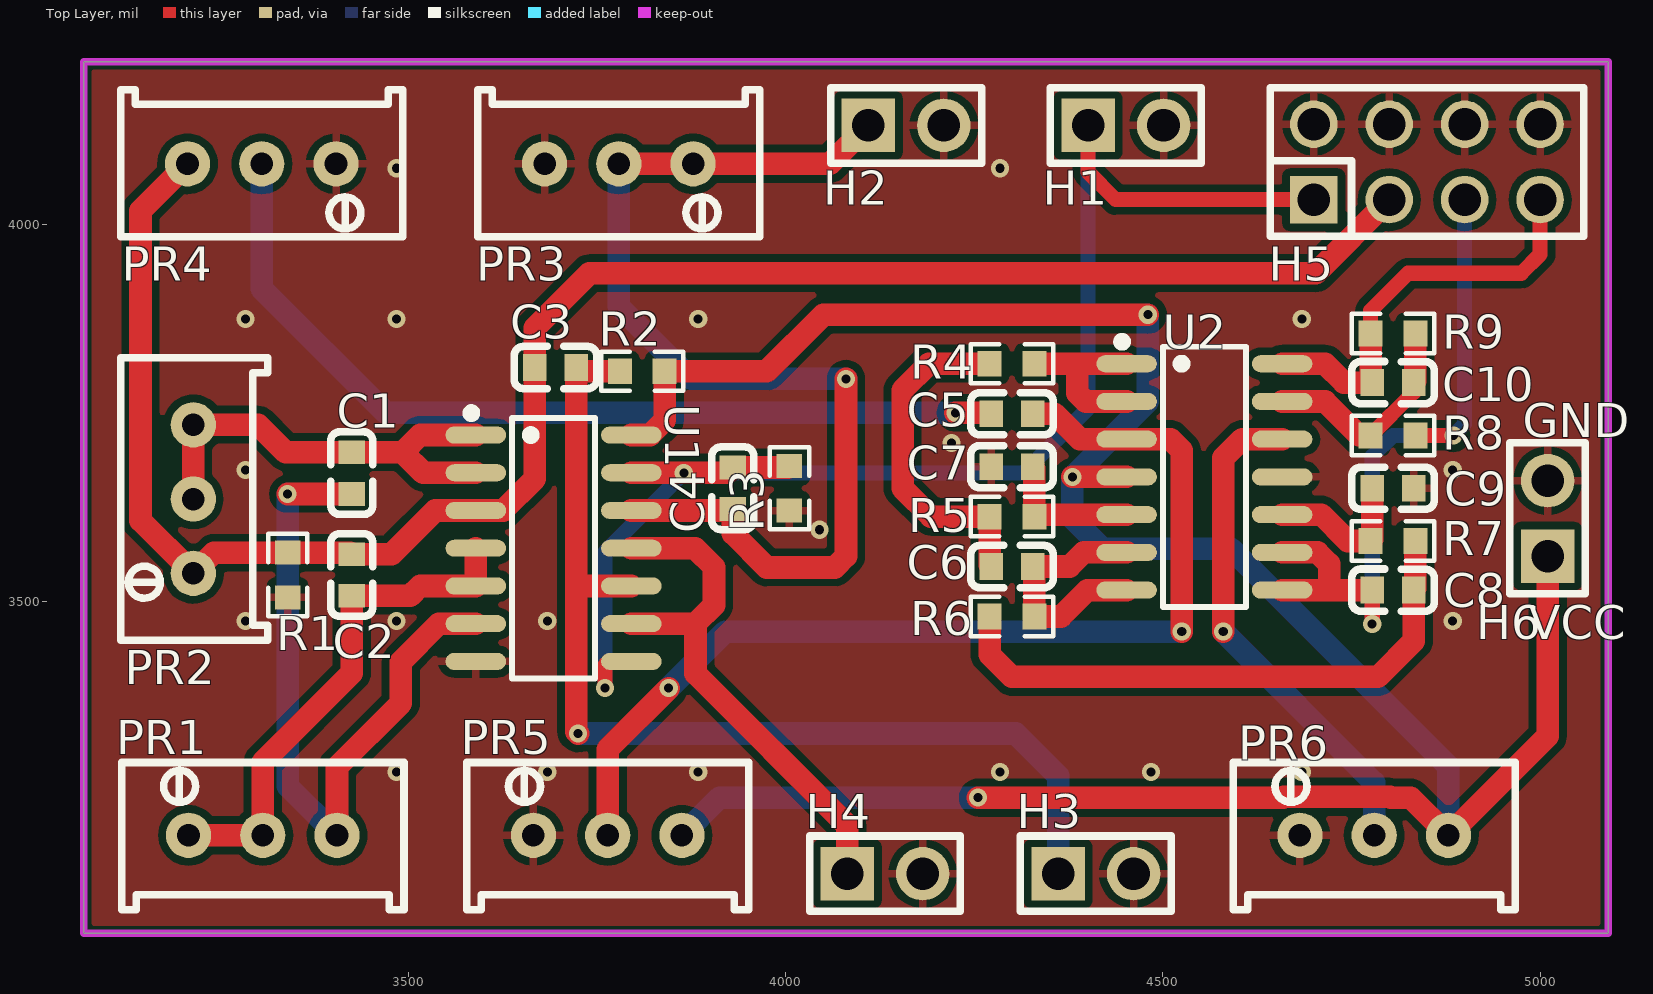
[diagram p0: Top Layer view]
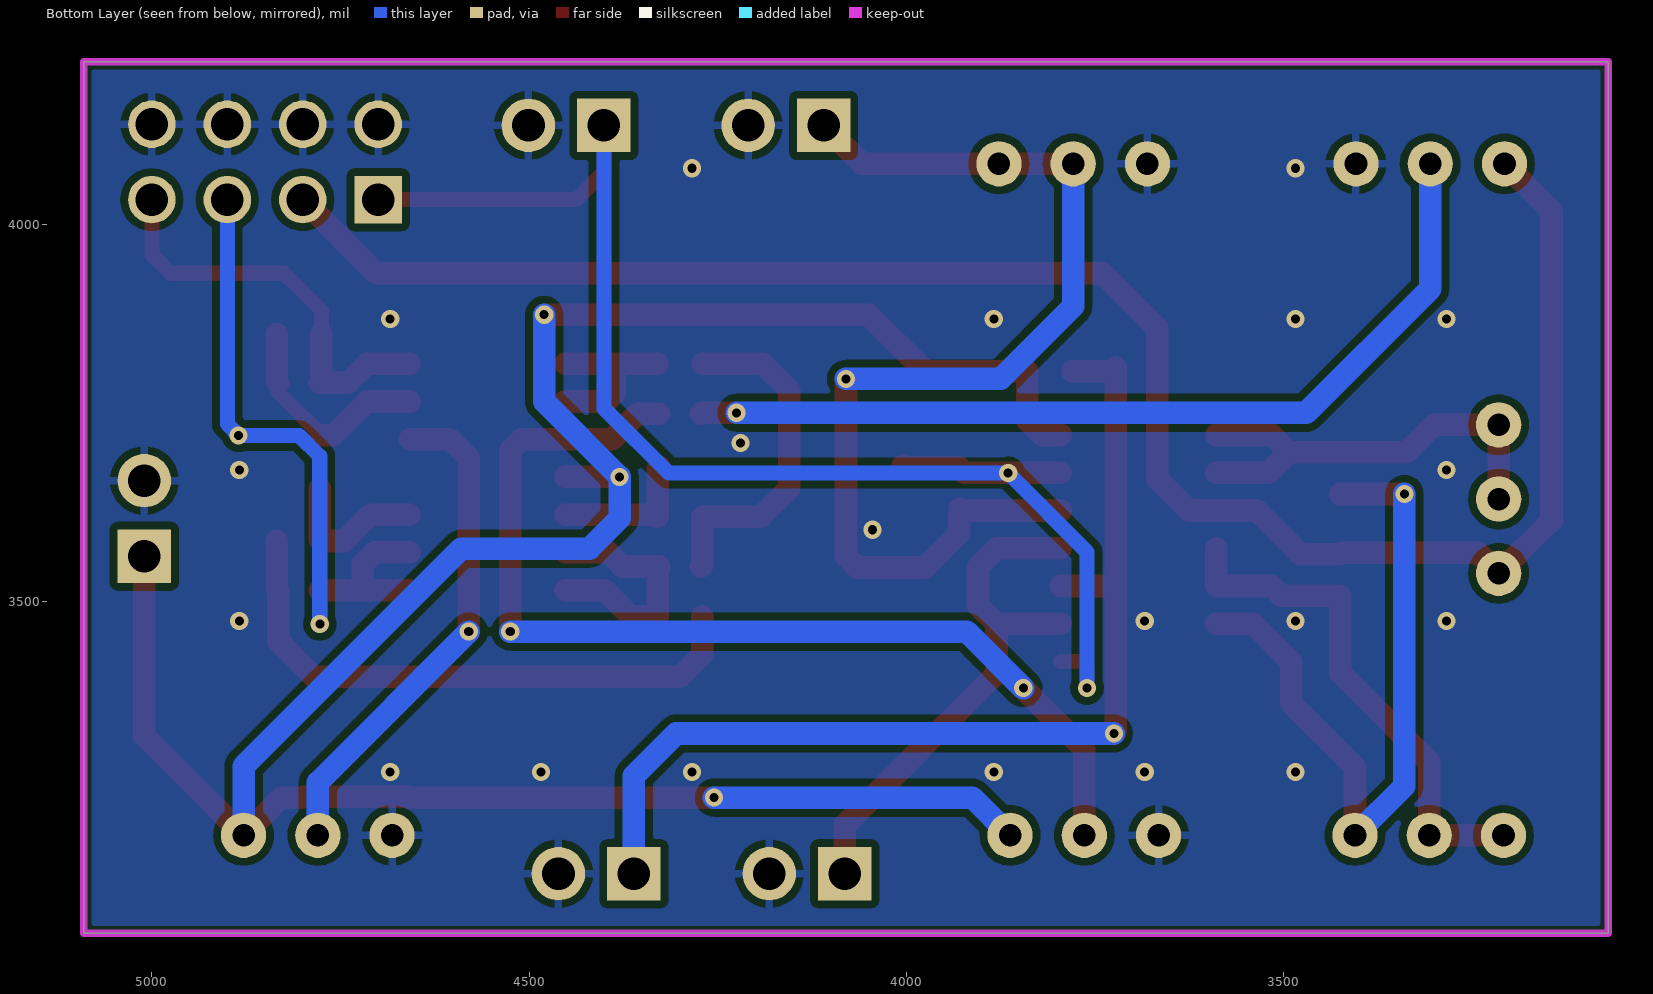
[diagram p1: Bottom Layer view, seen from below]
# Altium PCB MISC89095.pcbdoc
Units mil, origin at the board's own origin, x right, y up, seen from the top; angles counter-clockwise.
Board outline 2020 x 1155 mil, 2 copper layers (Top Layer, Bottom Layer), stack 62.206 mil thick; 33 components, 22 nets, 102 pads, 34 vias.

## Layer stack, top to bottom
Top Solder Mask Layer: solder mask 0.394, Dk 3.3
Top Layer: signal copper 1.379
Dielectric1: surface 59.449, FR4, Dk 4.5
Bottom Layer: signal copper 1.378
Bottom Solder Mask Layer: solder mask 0.394, Dk 3.3

## Board outline
3070,4215 3070,3060 5090,3060 5090,4215

## Design rules (kind name [scope] priority, off if disabled: settings)
BoardOutlineClearance copperThickness2oz_1 [All] p2 off: genericclearance=7.99 ignorepadtopadclearanceinfootprint=FALSE except(0: Arc-SplitContinuation Track-SplitContinuation SMDPad-SplitContinuation THPad-SplitContinuation Via-SplitContinuation Fill-SplitContinuation Region-SplitContinuation Poly-SplitContinuation Text-SplitContinuation Hole-SplitContinuation; 5.98: Arc-CutoutEdge SMDPad-CutoutEdge THPad-CutoutEdge Via-CutoutEdge Fill-CutoutEdge Region-CutoutEdge Text-CutoutEdge; 6.93: Hole-OutlineEdge Hole-CutoutEdge; 10: Poly-OutlineEdge Poly-CutoutEdge; 11.81: Arc-OutlineEdge Track-OutlineEdge SMDPad-OutlineEdge THPad-OutlineEdge Via-OutlineEdge Fill-OutlineEdge Region-OutlineEdge Text-OutlineEdge Track-CutoutEdge)
BoardOutlineClearance copperThickness1oz_1 [All] p4: genericclearance=4.02 ignorepadtopadclearanceinfootprint=FALSE except(0: Arc-SplitContinuation Track-SplitContinuation SMDPad-SplitContinuation THPad-SplitContinuation Via-SplitContinuation Fill-SplitContinuation Region-SplitContinuation Poly-SplitContinuation Text-SplitContinuation Hole-SplitContinuation; 6: SMDPad-CutoutEdge THPad-CutoutEdge Via-CutoutEdge Fill-CutoutEdge Region-CutoutEdge Text-CutoutEdge; 6.93: Hole-OutlineEdge Hole-CutoutEdge; 10: Poly-OutlineEdge Poly-CutoutEdge; 11.8: Arc-OutlineEdge Track-OutlineEdge SMDPad-OutlineEdge THPad-OutlineEdge Via-OutlineEdge Fill-OutlineEdge Region-OutlineEdge Text-OutlineEdge; 11.81: Arc-CutoutEdge Track-CutoutEdge)
Clearance copperThickness2oz [All] p1 off: gap=7.99 ignorepadtopadclearanceinfootprint=FALSE except(5.98: SMDPad-Track SMDPad-SMDPad THPad-Track SMDPad-THPad THPad-THPad Track-Via SMDPad-Via THPad-Via Via-Via Fill-Track Region-Track Fill-SMDPad Region-SMDPad Fill-THPad Region-THPad Fill-Via Region-Via Fill-Fill Fill-Region Region-Region Arc-Track Arc-SMDPad Arc-THPad Arc-Via Fill-Arc Region-Arc Arc-Arc Text-Track SMDPad-Text Text-THPad Text-Via Fill-Text Region-Text Arc-Text Text-Text; 6.93: Hole-Track Hole-SMDPad Hole-THPad Hole-Via Fill-Hole Region-Hole Hole-Arc Hole-Text; 10: Poly-Track Poly-SMDPad Poly-THPad Poly-Via Poly-Fill Poly-Region Poly-Poly Poly-Arc Poly-Text Poly-Hole)
Clearance copperThickness1oz [All] p3: gap=4.02 ignorepadtopadclearanceinfootprint=FALSE except(5.98: SMDPad-Track SMDPad-SMDPad THPad-Track SMDPad-THPad THPad-THPad Track-Via SMDPad-Via THPad-Via Via-Via Fill-Track Region-Track Fill-SMDPad Region-SMDPad Fill-THPad Region-THPad Fill-Via Region-Via Fill-Fill Fill-Region Region-Region; 6: Arc-Track Arc-SMDPad Arc-THPad Arc-Via Fill-Arc Region-Arc Arc-Arc Text-Track SMDPad-Text Text-THPad Text-Via Fill-Text Region-Text Arc-Text Text-Text; 6.93: Hole-Track Hole-SMDPad Hole-THPad Hole-Via Fill-Hole Region-Hole Hole-Arc Hole-Text; 10: Poly-Track Poly-SMDPad Poly-THPad Poly-Via Poly-Fill Poly-Region Poly-Poly Poly-Arc Poly-Text Poly-Hole)
Creepage creepage [All] p1: checkdistance=0 ignoreinternallayers=TRUE applytopolygonpour=TRUE
DiffPairsRouting differentialPair [All] p1: maxlimit=6 minlimit=6 mostfreqgap=6 toplayer_minwidth=5 toplayer_prefwidth=10 toplayer_maxwidth=100 toplayer_mingap=6 toplayer_prefgap=6 toplayer_maxgap=6 bottomlayer_minwidth=5 bottomlayer_prefwidth=10 bottomlayer_maxwidth=100 bottomlayer_mingap=6 bottomlayer_prefgap=6 bottomlayer_maxgap=6 maxuncoupledlength=10
HoleToHoleClearance otherClearance [All] p1: gap=11.81 allowstackedmicrovias=TRUE
Length netLength [All] p1: minlimit=0 maxlimit=0
MatchedLengths netLengthTolerance [All] p1: tolerance=1000
PasteMaskExpansion pasteMaskExpansion [All] p1: expansion=0
PlaneConnect innerPlane [All] p1: planeconnectstyle=Relief reliefexpansion=20 reliefentries=4 reliefconductorwidth=10 reliefairgap=10
PolygonConnect copperRegion [(InNet('GND'))] p1: connectstyle=Relief reliefconductorwidth=10 reliefentries=4 polygonreliefangle="90 Angle" airgapwidth=10 via.connectstyle=Relief via.reliefconductorwidth=10 via.reliefentries=4 via.polygonreliefangle="90 Angle" via.airgapwidth=10
RoutingVias viaSize [All] p1: holewidth=12.01 width=24.02 viastyle="Through Hole" minholewidth=11.81 minwidth=19.68 maxholewidth=248.03 maxwidth=393.7
SolderMaskExpansion solderMaskExpansion [IsVia] p1: expansion=-1000 istentingtop=TRUE
SolderMaskExpansion solderMaskExpansion [All] p2: expansion=2 istentingtop=FALSE
Width copperThickness2oz_2 [All] p1 off: maxlimit=100 minlimit=8 preferedwidth=10
Width copperThickness1oz_2 [All] p2: maxlimit=100 minlimit=5 preferedwidth=10

## Components (designator, comment, footprint, x,y, rotation, side; value= is the part's Value field where it differs from the comment)
C1 "22nF" C0603 3425,3670 r270 top
C2 "22nF" C0603 3425,3535 r270 top
C3 "100PF" C0603 3695,3810 r0 top
C4 "1nF" C0603 3930,3650 r90 top
C5 "100nF" C0603 4300,3748.79 r0 top
C6 "100pF" C0603 4300,3546.21 r0 top
C7 "100pF" C0603 4300,3678.63 r0 top
C8 "100pF" C0603 4805,3515 r180 top
C9 "80pF" C0603 4805,3650 r180 top
C10 "500pF" C0603 4805,3790 r0 top
H1 "" HDR-TH_2P-P2.54-V-M-1 4450.89,4130.9 r0 top
H2 "" HDR-TH_2P-P2.54-V-M-1 4159.66,4130.9 r0 top
H3 "" HDR-TH_2P-P2.54-V-M-1 4411.1,3139.1 r0 top
H4 "" HDR-TH_2P-P2.54-V-M-1 4131.7,3139.1 r0 top
H5 "" HDR-TH_8P-P2.54-V-F-R2-C4-S2.54-1 4850,4082.47 r0 top
H6 "" HDR-TH_2P-P2.54-V-M-1 5010,3610 r90 top
PR1 "10kΩ" R_3296 3307,3195 r0 top
PR2 "10kΩ" R_3296 3210,3635.65 r90 top
PR3 "20kΩ" R_3296 3778.93,4075 r180 top
PR4 "10kΩ" R_3296 3305.7,4075 r180 top
PR5 "10kΩ" R_3296 3764.1,3195 r0 top
PR6 "100kΩ" R_3296 4780,3195 r0 top
R1 "1K" R0603 3340,3535 r90 top
R2 "10K" R0603 3810,3805 r0 top
R3 "1K" R0603 4005,3650 r90 top
R4 "100K" R0603 4300,3815 r180 top
R5 "100K" R0603 4300,3612.42 r0 top
R6 "200K" R0603 4300,3480 r180 top
R7 "100K" R0603 4805,3580 r180 top
R8 "40K" R0603 4805,3720 r180 top
R9 "100K" R0603 4805,3855 r180 top
U1 "SN74LS00DG4" SOIC-14_L8.7-W3.9-P1.27-LS6.0-BL 3692.45,3570.51 r270 top
U2 "LM324DT" SOIC-14_L8.7-W3.9-P1.27-LS6.0-BL 4555,3665 r270 top

## Footprints (in the part's own frame and the unit in brackets; to place one, negate y for a bottom-side part, rotate by r counter-clockwise, add the part's x,y. Pads: shape width x height; smd on the part's side, far side on the other; paste and mask are expansions set on the pad)
C0603 [mm]
  rect 0.8x0.9 smd: 1(-0.7,0) 2(0.7,0)
  silkscreen extent -1.39,-0.71 1.39,0.71
HDR-TH_2P-P2.54-V-M-1 [mm]
  rect 1.8x1.8 hole 1.1: 1(-1.27,0)
  round 1.8 hole 1.1: 2(1.27,0)
  silkscreen extent -2.54,-1.27 2.54,1.27
HDR-TH_8P-P2.54-V-F-R2-C4-S2.54-1 [mm]
  rect 1.6x1.6 hole 1.1: 1(-3.81,-1.27)
  round 1.6 hole 1.1: 2(-3.81,1.27) 3(-1.27,-1.27) 4(-1.27,1.27) 5(1.27,-1.27) 6(1.27,1.27) 7(3.81,-1.27) 8(3.81,1.27)
  silkscreen extent -5.28,-2.5 5.28,2.5
R0603 [mil]
  rect 31.75x34.02 smd paste-3937.01 mask+2: 1(-29.66,0) 2(29.66,0)
  silkscreen extent -55,-26 55,26
R_3296 [mil]
  round 60 hole 30 paste+0 mask+2: 1(-98.4,-5) 2(0,-5) 3(98.4,-5)
  silkscreen extent -187,-103 187,92
SOIC-14_L8.7-W3.9-P1.27-LS6.0-BL [mil]
  oval 22.6x80.24 smd: 1(-150,-103.11) 2(-100,-103.11) 3(-50,-103.11) 4(0,-103.11) 5(50,-103.11) 6(100,-103.11) 7(150,-103.11) 8(150,103.11) 9(100,103.11) 10(50,103.11) 11(0,103.11) 12(-50,103.11) 13(-100,103.11) 14(-150,103.11)
  silkscreen extent -185,-115 172,55

## Via types
v1: diameter 24.02, hole 12, Top Layer to Bottom Layer, 34 vias

## Nets (pads, with @x,y where several pads share a name; then routed paths per layer and width w, separated by ;. In a path a pad name is that pad's centre, name@x,y a point inside that pad or via, vN(x,y) a via of type N, cw(c..) or ccw(c..) an arc to the next point about the centre after c; other vN are vias at no path point)
$1N1: C1.1 PR2.2 PR2.3 U1.1 U1.2 | length 605.3
  Top Layer w30: PR2.2 PR2.3 3300.95,3734.05 3337.44,3697.56 C1.1 3492.56,3697.56 ; U1.2 3519.61,3670.51 3492.56,3697.56 ; U1.1 3515.51,3720.51 3492.56,3697.56
$1N4: C2.2 PR1.1 PR1.2 U1.4 U1.5 | length 684.5
  Top Layer w30: PR1.1 PR1.2 3307,3287 3425,3405 C2.2 3502.44,3507.44 3515.51,3520.51 U1.5 U1.4
$1N6: C1.2 PR1.3 U1.6 | length 949.8
  Top Layer w30: v1(3340,3642.44) C1.2 ; PR1.3 3405.4,3280.4 3490,3365 3490,3420 3540.51,3470.51 U1.6
  Bottom Layer w30: v1(3340,3642.44) 3340,3255.4 PR1.3
$1N12: C3.2 H3.1 R2.1 U1.10 | length 1408
  Top Layer w30: v1(3725,3325) 3722.56,3327.44 3722.56,3520.51 ; R2.1 3727.56,3805 C3.2 3722.56,3520.51 ; U1.10 3722.56,3520.51
  Bottom Layer w30: v1(3725,3325) 4305,3325 4361.1,3268.9 H3.1
$1N16: H4.1 U1.9 U1.11 | length 704.6
  Top Layer w30: U1.9 3880.51,3470.51 ; U1.11 3879.99,3570.51 3905,3545.5 3905,3495 3880.51,3470.51 ; H4.1 4081.7,3203.3 3880.51,3404.49 3880.51,3470.51
$1N20: C4.1 H2.1 PR3.1 PR3.2 U1.12 | length 1459.1
  Top Layer w30: PR3.2 PR3.1 4058.76,4080 H2.1 ; U1.12 3928.08,3620.51 C4.1 3930,3590 3975,3545 4065,3545 4080,3560 v1(4080,3795)
  Bottom Layer w30: PR3.2 3778.93,3891.07 3875,3795 v1(4080,3795)
$1N21: C4.2 H1.1 H5.1 R3.2 U1.8 U1.13 | length 1931.7
  Top Layer w20: v1(3760.56,3385) 3760.56,3415.56 3765.51,3420.51 U1.8 ; H1.1 4400.89,4069.11 4437.52,4032.47 H5.1
  Top Layer w30: U1.13 3922.96,3670.51 C4.2 4002.9,3677.56 R3.2
  Bottom Layer w20: v1(3760.56,3385) 3760.56,3565.56 v1(3865,3670) 4315,3670 4400.89,3755.89 H1.1
$1N27: C5.1 PR4.2 | length 1201
  Top Layer w30: v1(4225,3750) 4271.23,3750 C5.1
  Bottom Layer w30: PR4.2 3305.7,3914.3 3470,3750 v1(4225,3750)
$1N28: C5.2 PR5.2 U2.3 | length 1397.2
  Top Layer w30: PR5.2 3764.1,3304.1 v1(3845,3385) ; C5.2 4356.21,3748.79 4390,3715 U2.3 4510,3715 4525,3700 v1(4525,3460)
  Bottom Layer w30: v1(3845,3385) 3920,3460 v1(4525,3460)
$1N33: R4.1 U2.1 U2.2 | length 231.1
  Top Layer w30: R4.1 4386.65,3815 ; U2.2 4397.52,3765 4386.65,3775.87 4386.65,3815 ; U2.1 4386.65,3815
$1N35: C6.2 R6.1 U2.6 U2.7 | length 335.9
  Top Layer w30: U2.7 4400,3515 4365,3480 R6.1 4329.66,3544.11 C6.2 4376.21,3546.21 4395,3565 U2.6
$1N36: C6.1 R4.2 R5.1 | length 457.8
  Top Layer w30: R4.2 4190,3815 4155,3780 4155,3650 4192.58,3612.42 R5.1 4270.34,3548.31 C6.1
$1N37: C7.2 R5.2 U2.5 | length 190.4
  Top Layer w30: C7.2 4329.66,3676.53 R5.2 4332.24,3615 U2.5
$1N39: C8.1 R6.2 R7.1 | length 777.9
  Top Layer w30: R6.2 4270.34,3429.66 4300,3400 4785,3400 4832.56,3447.56 C8.1 4834.66,3517.1 R7.1
$1N41: C9.2 R7.2 U2.10 | length 202.6
  Top Layer w30: U2.10 4710,3615 4745,3580 R7.2 4777.44,3582.1 C9.2
$1N43: C10.2 R8.2 R9.1 U2.13 | length 295.4
  Top Layer w20: R8.2 4832.56,3777.22 C10.2
  Top Layer w30: U2.13 4715,3765 4760,3720 R8.2 ; C10.2 4834.66,3792.1 R9.1
$1N44: C10.1 H5.7 R9.2 U2.14 | length 554
  Top Layer w20: R9.2 4775.34,3885.34 4825,3935 4975,3935 5000,3960 H5.7
  Top Layer w30: U2.14 4715,3815 4740,3790 C10.1 4775.34,3792.1 R9.2
$1N45: PR6.2 U2.12 | length 671.3
  Top Layer w30: v1(4580,3460) 4580,3690 4605,3715 U2.12
  Bottom Layer w30: v1(4580,3460) 4780,3260 PR6.2
$1N48: C8.2 H5.5 R8.1 U2.8 U2.9 | length 978
  Top Layer w20: v1(4777.44,3470) C8.2 ; R8.1 v1(4885,3720)
  Top Layer w30: U2.8 4720.29,3515 ; U2.9 4705,3565 4720.29,3549.71 4720.29,3515 ; C8.2 4720.29,3515
  Bottom Layer w20: v1(4777.44,3470) 4777.44,3692.44 4805,3720 v1(4885,3720) 4900,3735 H5.5
$1N49: C2.1 C3.1 H5.3 PR2.1 PR4.3 R1.2 U1.3 | length 2506.6
  Top Layer w30: PR4.3 3145,4017.7 3145,3607.25 PR2.1 3242.41,3564.66 R1.2 3422.9,3564.66 C2.1 3477.56,3562.56 3535.51,3620.51 U1.3 3625.51,3620.51 3667.44,3662.44 C3.1 3667.44,3862.44 3740,3935 4702.52,3935 H5.3
GND: C7.1 C9.1 H1.2 H2.2 H3.2 H4.2 H5.2 H5.4 H5.6 H5.8 H6.2 PR3.3 PR4.1 PR5.1 PR6.1 R1.1 R3.1 U1.7 U2.11
  other v1: 3484.1,3274.1 3684.1,3274.1 3884.1,3274.1 4284.1,3274.1 4484.1,3274.1 4684.1,3274.1 3284.1,3474.1 3484.1,3474.1 3684.1,3474.1 4884.1,3474.1 4045,3595 3284.1,3674.1 4884.1,3674.1 4220,3710 3284.1,3874.1 3484.1,3874.1 3884.1,3874.1 4684.1,3874.1 3484.1,4074.1 4284.1,4074.1
VCC: H6.1 PR5.3 PR6.3 R2.2 U1.14 U2.4 | length 3380.6
  Top Layer w30: U1.14 3820.17,3720.51 3839.66,3740 R2.2 3975,3805 4050,3880 v1(4480,3880) ; v1(4255,3240) 4659.5,3240 4660.48,3240.98 4801.12,3240.98 4802.1,3240 4828.4,3240 PR6.3 5010,3321.6 H6.1 ; v1(4380,3665) U2.4
  Bottom Layer w30: PR5.3 3912.5,3240 v1(4255,3240) ; v1(4480,3880) 4480,3765 v1(4380,3665) 4380,3610 4420,3570 4590,3570 4878.4,3281.6 PR6.3

## Polygon pours and split planes (outlines as drawn)
GND on Top Layer (solid, remove dead copper, pour order 0): 3000,4300 3000,3000 5190,3000 5190,4300
GND on Bottom Layer (solid, remove dead copper, pour order 2): 3045,4270 3045,3000 5195,3000 5195,4270

## Keep-outs
Board Outline Layer:
  the board outline again, w10

## Silkscreen, mask and mechanical layers (free items; w line width, h text height)
Top Silkscreen Layer:
  text "GND" at 4977.15,3717.5 h45
  text "VCC" at 4985,3450 h45